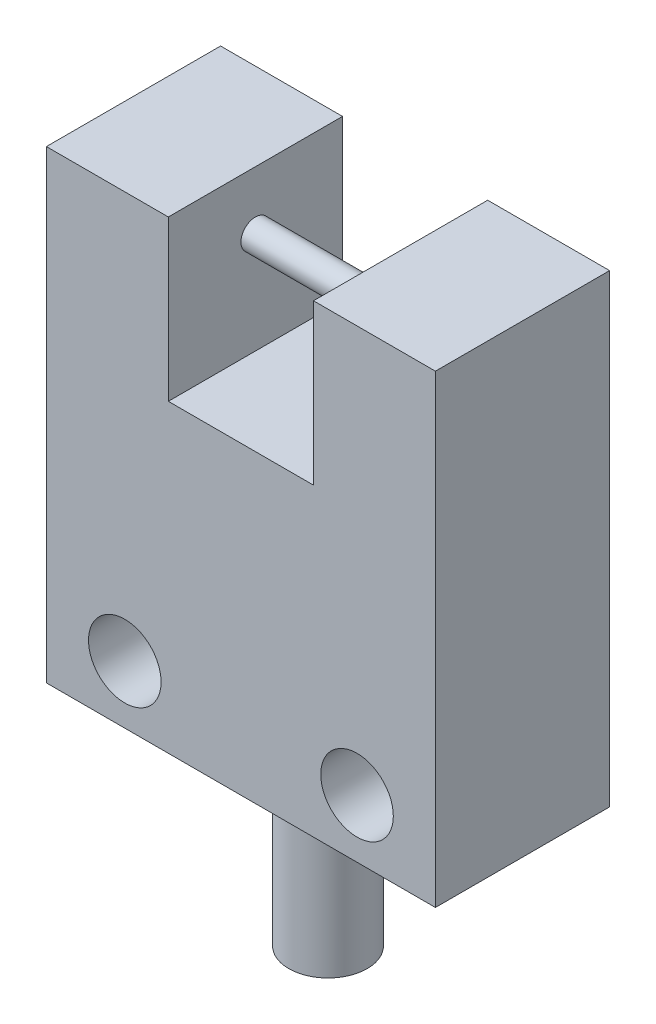
from build123d import *

# Parameters (mm, degrees)
SKETCH1_W                  = 13.4
SKETCH1_H                  = 16
BOSS_EXTRUDE1_DEPTH        = 3
SKETCH2_W                  = 5
SKETCH2_H                  = 5.5
CUT_EXTRUDE1_DEPTH         = 13.037026211
SKETCH3_R                  = 1.35
BOSS_EXTRUDE2_DEPTH        = 6
F_2_5_2_5_DIAMETER_HOLE1_D = 2.5
SKETCH6_R                  = 0.5
BOSS_EXTRUDE3_DEPTH        = 5


with BuildPart() as part:
    # Sketch1 → Boss-Extrude1 (new, symmetric)
    with BuildSketch(Plane.XY):
        Rectangle(SKETCH1_W, SKETCH1_H)
    extrude(amount=BOSS_EXTRUDE1_DEPTH, both=True)

    # Sketch2 → Cut-Extrude1 (cut, through all)
    with BuildSketch(Plane.XY.offset(3)):
        with Locations((0, 5.25)):
            Rectangle(SKETCH2_W, SKETCH2_H)
    extrude(amount=-CUT_EXTRUDE1_DEPTH, mode=Mode.SUBTRACT)

    # Sketch3 → Boss-Extrude2 (add)
    with BuildSketch(Plane.XZ.offset(8)):
        with Locations(Location((0, 0, 0), (0, 0, 90))):
            Circle(SKETCH3_R)
    extrude(amount=BOSS_EXTRUDE2_DEPTH)

    # Ø2.5 (2.5) Diameter Hole1 (through all)
    with Locations(Plane.XY.offset(3)):
        with Locations((-4, -6), (4, -6)):
            Hole(F_2_5_2_5_DIAMETER_HOLE1_D / 2)

    # Sketch6 → Boss-Extrude3 (add)
    with BuildSketch(Plane.ZY.offset(-2.5)):
        with Locations(Location((0, 6, 0), (0, 0, 90))):
            Circle(SKETCH6_R)
    extrude(amount=BOSS_EXTRUDE3_DEPTH)


solid = part.part
